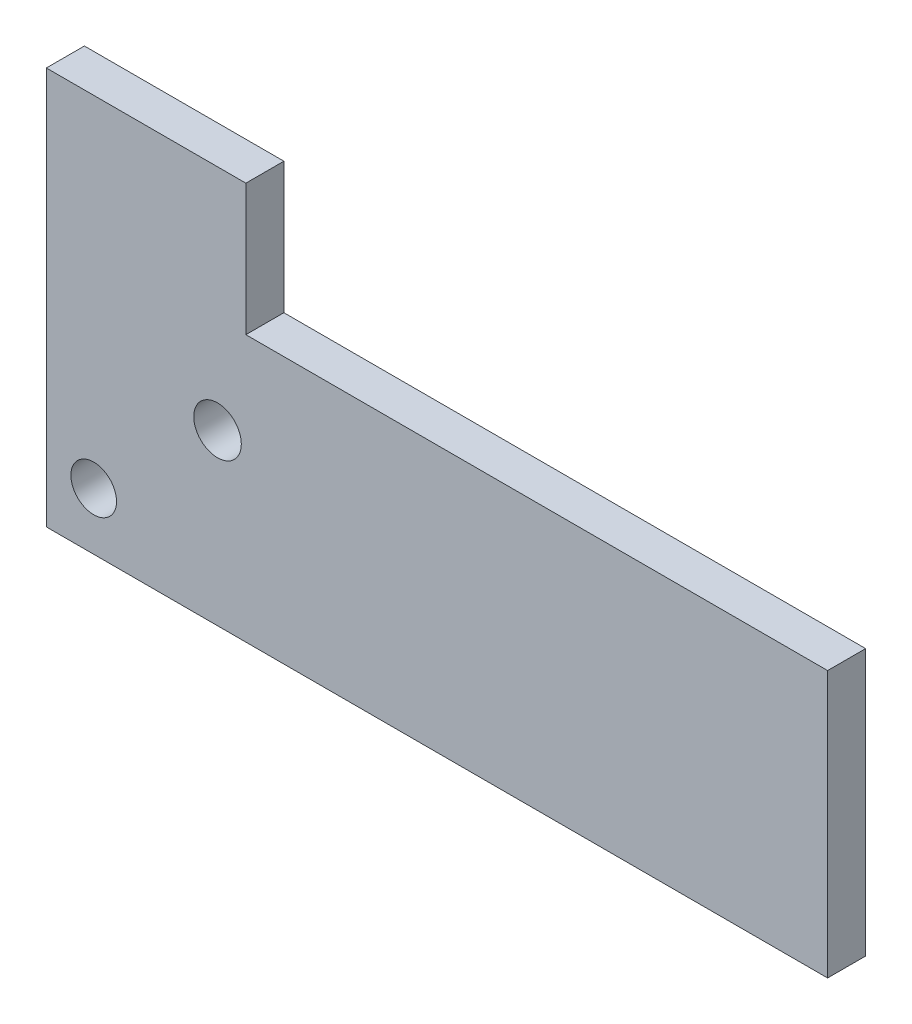
SolidWorks part; units mm, degrees
ref_plane "Front Plane" through (0, 0, 0) normal (0, 0, 1) x (1, 0, 0)
ref_plane "Top Plane" through (0, 0, 0) normal (0, 1, 0) x (1, 0, 0)
ref_plane "Right Plane" through (0, 0, 0) normal (1, 0, 0) x (0, 0, -1)
sketch "Sketch1" plane through (0, 0, 0) normal (0, 0, 1) x (1, 0, 0)
  line L0 (7.55, 34.5) -> (7.55, -70)
  line L2 (60, 34.5) -> (60, 0)
  line L3 (60, 0) -> (137.7273, 0)
  line L4 (7.55, -70) -> (212.9421, -70)
  line L7 (212.9421, -70) -> (212.9421, 0)
  line L8 (212.9421, 0) -> (137.7273, 0)
  line L10 (60, 34.5) -> (7.55, 34.5)
  circle A0 centre (20, -55) radius 6
  circle A1 centre (52.55, -25.5) radius 6.25
  dimension "D5" = 12
extrude "Boss-Extrude1" add sketch "Sketch1" along normal blind 10
